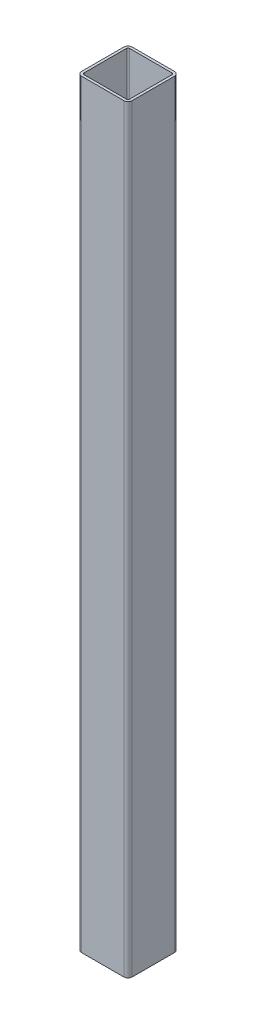
SolidWorks part; units mm, degrees
material "Q235B"
ref_plane "Front Plane" through (0, 0, 0) normal (0, 0, 1) x (1, 0, 0)
ref_plane "Top Plane" through (0, 0, 0) normal (0, 1, 0) x (1, 0, 0)
ref_plane "Right Plane" through (0, 0, 0) normal (1, 0, 0) x (0, 0, -1)
other "Configuration Table"
sketch "Sketch1" plane through (0, 0, 0) normal (0, 1, 0) x (1, 0, 0)
  line L0 (-54, -50) -> (-54, 50)
  line L1 (-50, -60) -> (50, -60)
  line L2 (-60, -50) -> (-60, 50)
  line L3 (-50, 60) -> (50, 60)
  line L4 (60, -50) -> (60, 50)
  line L5 (-60, -60) -> (60, 60) construction
  line L6 (-60, 60) -> (60, -60) construction
  line L7 (-50, 54) -> (50, 54)
  line L8 (54, -50) -> (54, 50)
  line L9 (-50, -54) -> (50, -54)
  arc A0 (-50, -60) -> (-60, -50) centre (-50, -50) cw
  arc A1 (50, -60) -> (60, -50) centre (50, -50) ccw
  arc A2 (50, 60) -> (60, 50) centre (50, 50) cw
  arc A3 (-60, 50) -> (-50, 60) centre (-50, 50) cw
  arc A4 (-54, 50) -> (-50, 54) centre (-50, 50) cw
  arc A5 (50, 54) -> (54, 50) centre (50, 50) cw
  arc A6 (50, -54) -> (54, -50) centre (50, -50) ccw
  arc A7 (-50, -54) -> (-54, -50) centre (-50, -50) cw
  point P0 (0, 0)
  dimension "D3" = 10
  dimension "D1" = 120
  dimension "D2" = 120
  dimension "D4" = 6
extrude "Boss-Extrude1" add sketch "Sketch1" along normal blind 1800
